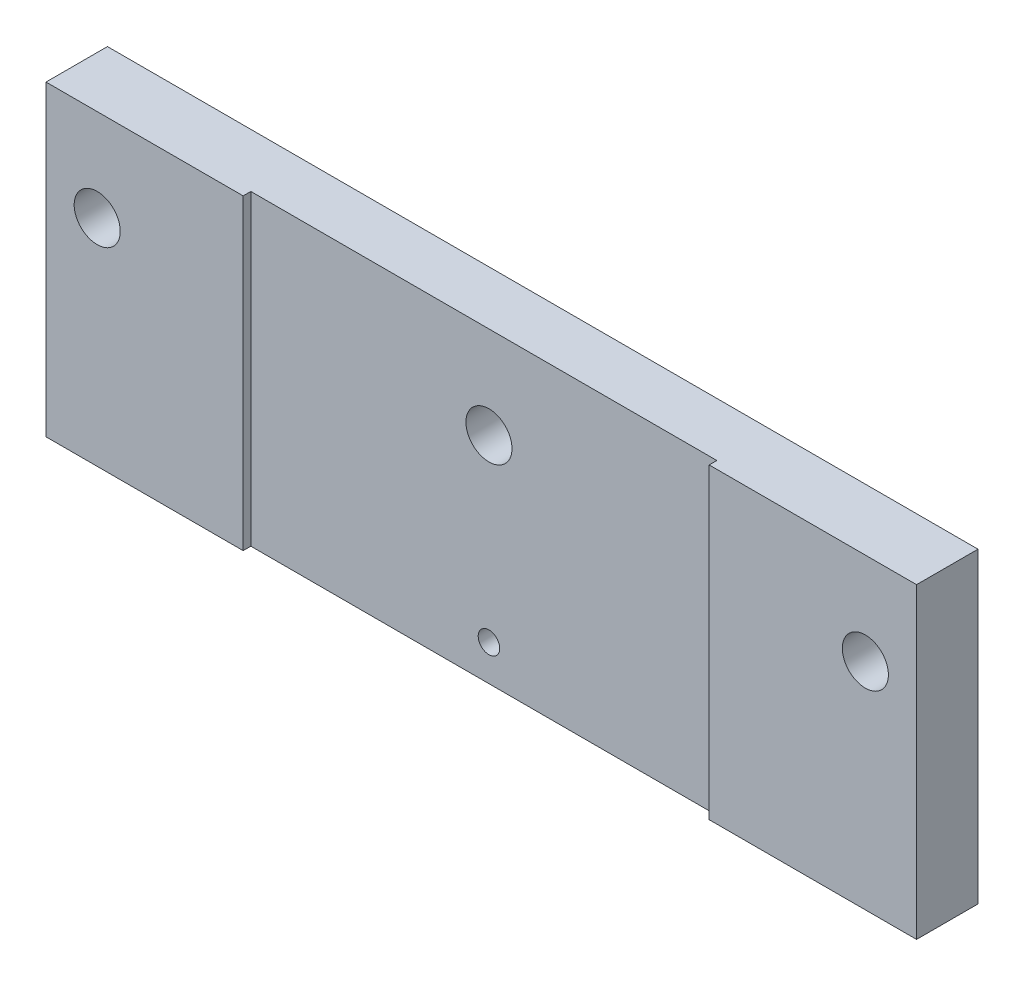
SolidWorks part; units mm, degrees
ref_plane "前视基准面" through (0, 0, 0) normal (0, 0, 1) x (1, 0, 0)
ref_plane "上视基准面" through (0, 0, 0) normal (0, 1, 0) x (1, 0, 0)
ref_plane "右视基准面" through (0, 0, 0) normal (1, 0, 0) x (0, 0, -1)
sketch "草图1" plane through (0, 0, 0) normal (0, 0, 1) x (1, 0, 0)
  line L1 (-85, -30) -> (85, -30)
  line L2 (-85, -30) -> (-85, 30)
  line L3 (-85, 30) -> (85, 30)
  line L4 (85, -30) -> (85, 30)
  line L5 (-85, -30) -> (85, 30) construction
  line L6 (-85, 30) -> (85, -30) construction
  circle A0 centre (-75, 12) radius 4.5
  circle A2 centre (75, 12) radius 4.5
  circle A3 centre (0, 12) radius 4.5
  point P0 (0, 0)
extrude "凸台-拉伸1" add sketch "草图1" along normal mid plane 12
sketch "草图2" plane through (0, 0, 6) normal (0, 0, 1) x (1, 0, 0)
  line L0 (85, 30) -> (-85, 30) construction
  line L1 (44.5, 30) -> (-46.5, 30)
  line L2 (44.5, 30) -> (44.5, -30)
  line L3 (44.5, -30) -> (-46.5, -30)
  line L4 (-46.5, 30) -> (-46.5, -30)
  line L5 (-85, -30) -> (85, -30) construction
extrude "切除-拉伸1" cut sketch "草图2" against normal blind 1.5
hole_wizard "M5 螺纹孔1" positions "3D草图1" profile "草图3" tap size "M5" standard "GB" end condition up to next
sketch3d "3D草图1"
  line L3 (0, -23, -6) -> (0, -30, -6)
  line L4 (-85, -30, -6) -> (85, -30, -6) construction
  point P0 (0, -23, -6)
  dimension "D1" = 7
sketch "草图3" plane through (0, -23, -6) normal (1, 0, 0) x (0, 1, 0)
  line L0 (0, 0) -> (0, 10.5)
  line L1 (0, 10.5) -> (2.1, 10.5)
  line L2 (2.1, 10.5) -> (2.1, 0.425)
  line L3 (2.1, 0.425) -> (2.525, 0)
  line L5 (2.525, 0) -> (0, 0)
  line L6 (-2.1, 0.425) -> (-2.525, 0) construction
  line L11 (0, -6.35) -> (0, 107.95) construction
  dimension "通孔螺纹孔钻头直径" = 4.2
  dimension "通孔螺纹孔钻头深度" = 10.5
  dimension "近端锥形沉头孔直径" = 5.05
  dimension "近端锥形沉头孔角度" = 90
cosmetic thread "孔螺蚊线1" parameters "D2"=5
sketch "草图4" plane through (0, 0, -6) normal (0, 0, -1) x (-1, 0, 0)
  circle A0 centre (0, -23) radius 3
  dimension "D1" = 6
extrude "切除-拉伸2" [suppressed] cut sketch "草图4" against normal blind 2
equation "\"D2@草图2\"=\"D1@草图2\"+2"
equation "\"D2@草图1\"=\"D5@草图1\""
